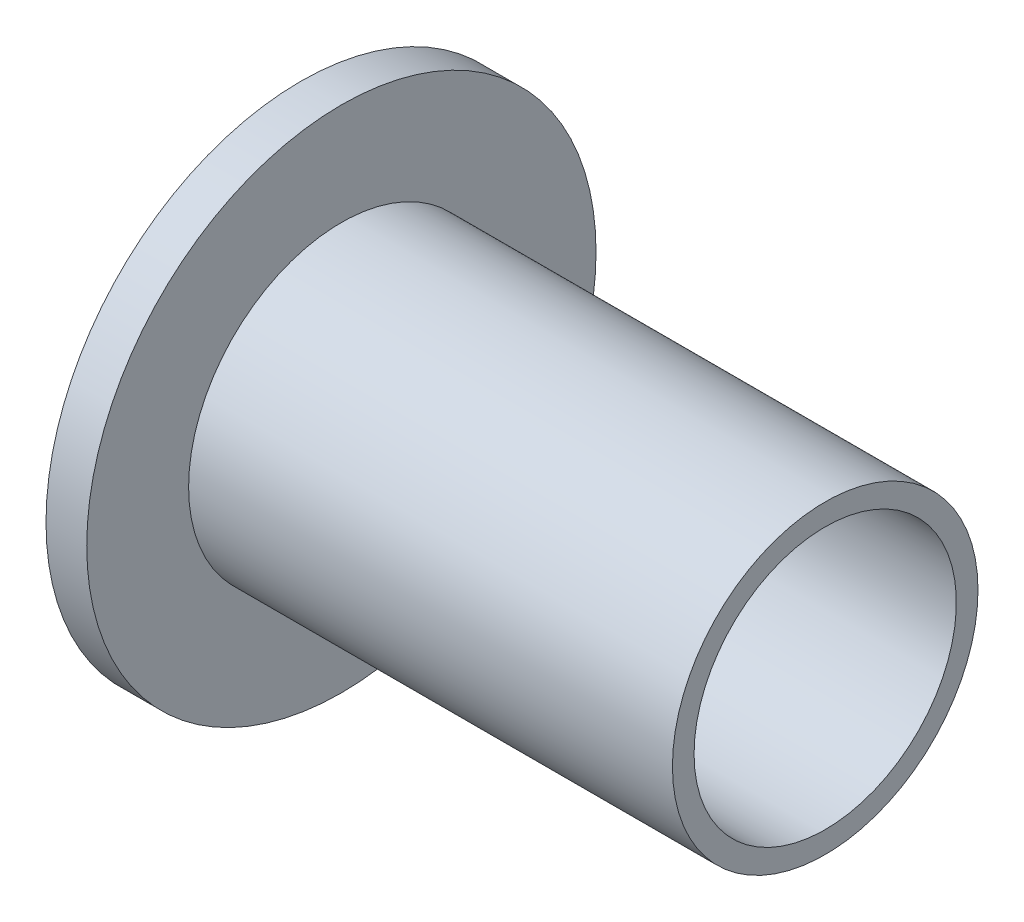
from build123d import *


with BuildPart() as part:
    # 草图1 → 旋转1 (revolve)
    with BuildSketch(Plane.XY, mode=Mode.PRIVATE) as revolve_1_sk:
        Polygon((0, 5.15), (0, 10), (1.6, 10), (1.6, 6), (20.6, 6), (20.6, 5.15), align=None)
    revolve(revolve_1_sk.sketch.rotate(Axis((0, 0, 0), (1, 0, 0)), 90), axis=Axis((0, 0, 0), (1, 0, 0)))


solid = part.part
